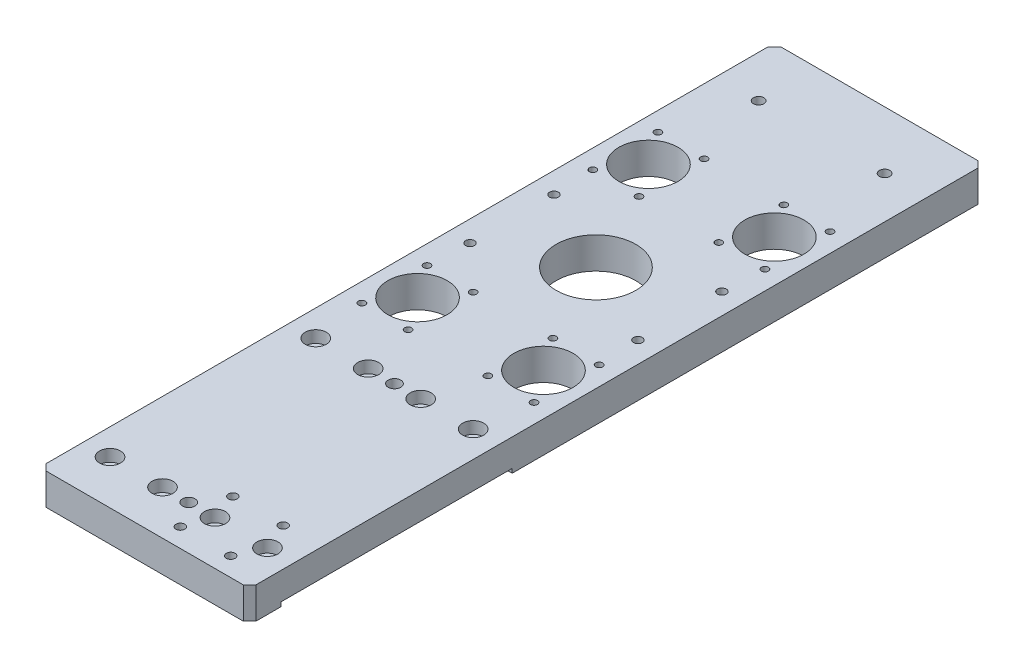
SolidWorks part; units mm, degrees
material "A6061 T6"
ref_plane "前视基准面" through (0, 0, 0) normal (0, 0, 1) x (1, 0, 0)
ref_plane "上视基准面" through (0, 0, 0) normal (0, 1, 0) x (1, 0, 0)
ref_plane "右视基准面" through (0, 0, 0) normal (1, 0, 0) x (0, 0, -1)
sketch "草图1" plane through (0, 0, 0) normal (0, 1, 0) x (1, 0, 0)
  line L1 (-50, 175) -> (50, 175)
  line L2 (-50, 175) -> (-50, -175)
  line L3 (-50, -175) -> (50, -175)
  line L4 (50, 175) -> (50, -175)
  line L5 (-50, 175) -> (50, -175) construction
  line L6 (-50, -175) -> (50, 175) construction
  point P0 (0, 0)
  dimension "D1" = 100
  dimension "D2" = 350
extrude "凸台-拉伸1" add sketch "草图1" along normal blind 15
sketch "草图3" plane through (0, 0, 0) normal (0, -1, 0) x (1, 0, 0)
  line L0 (-50, -175) -> (-50, 175) construction
  line L1 (-50, 160.1) -> (50, 160.1)
  line L2 (-50, 160.1) -> (-50, 49.9)
  line L3 (-50, 49.9) -> (50, 49.9)
  line L4 (50, 160.1) -> (50, 49.9)
  line L5 (50, 175) -> (50, -175) construction
  line L6 (-50, 175) -> (50, 175) construction
  dimension "D1" = 14.9
  dimension "D2" = 110.2
extrude "切除-拉伸1" cut sketch "草图3" against normal blind 2
hole_wizard "打孔尺寸(%根据)内六角圆柱头螺钉的类型1" positions "草图4" profile "草图5" counterbore size "M5" standard "GB"
sketch "草图4" plane through (0, 15, 0) normal (0, 1, 0) x (1, 0, 0)
  point P0 (-37.5, -154)
  point P3 (-12.5, -154)
  point P6 (12.5, -154)
  point P9 (37.5, -154)
  point P12 (-37.5, -56)
  point P15 (-12.5, -56)
  point P18 (12.5, -56)
  point P21 (37.5, -56)
sketch "草图5" plane through (-37.5, 15, 154) normal (1, 0, 0) x (0, 0, 1)
  line L0 (0, 0) -> (0, 16.6524)
  line L1 (0, 16.6524) -> (2.75, 15)
  line L2 (2.75, 15) -> (2.75, 5.7)
  line L3 (2.75, 5.7) -> (5, 5.7)
  line L4 (5, 5.7) -> (5, 0)
  line L5 (5, 0) -> (0, 0)
  line L10 (0, 16.6524) -> (-2.75, 15) construction
  line L11 (0, -6.35) -> (0, 107.95) construction
  dimension "孔直径" = 5.5
  dimension "孔深度" = 15
  dimension "柱形沉头孔直径" = 10
  dimension "柱形沉头孔深度" = 5.7
  dimension "导头角度" = 118
hole_wizard "大小mm 暗销孔1" positions "草图6" profile "草图7" hole size "Ø6.0" standard "GB"
sketch "草图6" plane through (0, 15, 0) normal (0, 1, 0) x (1, 0, 0)
  point P2 (0, -154)
  point P5 (0, -56)
sketch "草图7" plane through (0, 15, 154) normal (1, 0, 0) x (0, 0, 1)
  line L0 (0, 0) -> (0, 16.8026)
  line L1 (0, 16.8026) -> (3, 15)
  line L2 (3, 15) -> (3, 0)
  line L5 (3, 0) -> (0, 0)
  line L10 (0, 16.8026) -> (-3, 15) construction
  line L11 (0, -6.35) -> (0, 107.95) construction
  dimension "孔直径" = 6
  dimension "孔深度" = 15
  dimension "导头角度" = 118
sketch "草图8" plane through (0, 15, 0) normal (0, 1, 0) x (1, 0, 0)
  line L0 (-50, 175) -> (-50, -175) construction
  line L1 (50, 175) -> (-50, 175) construction
  circle A0 centre (0, 40) radius 19
  dimension "D1" = 38
  dimension "D2" = 50
  dimension "D3" = 135
extrude "切除-拉伸2" cut sketch "草图8" against normal blind 20
chamfer "倒角1" distance 3 angle 45 4 edges at (50, 7.5, -175) (-50, 7.5, -175) (50, 7.5, 175) (-50, 7.5, 175)
sketch "草图9" plane through (0, 15, 0) normal (0, 1, 0) x (1, 0, 0)
  line L0 (47, 175) -> (-47, 175) construction
  line L1 (50, -172) -> (50, 172) construction
  line L2 (-50, 172) -> (-50, -172) construction
  circle A0 centre (30, -15) radius 14.1
  circle A1 centre (30, 95) radius 14.1
  circle A3 centre (-30, -15) radius 14.1
  circle A4 centre (-30, 95) radius 14.1
  dimension "D1" = 80
  dimension "D2" = 110
  dimension "D3" = 28.2
  dimension "D4" = 20
  dimension "D5" = 28.2
  dimension "D6" = 20
extrude "切除-拉伸3" cut sketch "草图9" against normal blind 20
hole_wizard "大小mm 暗销孔2" positions "草图14" profile "草图15" hole size "Ø5.0" standard "GB"
sketch "草图14" plane through (0, 15, 0) normal (0, 1, 0) x (1, 0, 0)
  point P0 (30, 147.5)
  point P3 (-30, 147.5)
sketch "草图15" plane through (30, 15, -147.5) normal (1, 0, 0) x (0, 0, 1)
  line L0 (0, 0) -> (0, 21.5022)
  line L1 (0, 21.5022) -> (2.5, 20)
  line L2 (2.5, 20) -> (2.5, 0)
  line L5 (2.5, 0) -> (0, 0)
  line L10 (0, 21.5022) -> (-2.5, 20) construction
  line L11 (0, -6.35) -> (0, 107.95) construction
  dimension "孔直径" = 5
  dimension "孔深度" = 20
  dimension "导头角度" = 118
hole_wizard "M5 螺纹孔1" positions "草图18" profile "草图19" tap size "M5" standard "GB"
sketch "草图18" plane through (0, 0, 0) normal (0, -1, 0) x (-1, 0, 0)
  point P0 (40, 20)
  point P3 (-40, 20)
  point P6 (40, 60)
  point P9 (-40, 60)
sketch "草图19" plane through (-40, 0, -20) normal (1, 0, 0) x (0, 0, -1)
  line L0 (0, 0) -> (0, 21.2618)
  line L1 (0, 21.2618) -> (2.1, 20)
  line L2 (2.1, 20) -> (2.1, 0)
  line L5 (2.1, 0) -> (0, 0)
  line L10 (0, 21.2618) -> (-2.1, 20) construction
  line L11 (0, -6.35) -> (0, 107.95) construction
  dimension "螺纹孔钻头直径" = 4.2
  dimension "螺纹孔钻头深度" = 20
  dimension "导头角度" = 118
cosmetic thread "孔螺蚊线5" parameters "D1"=10, "D2"=5
cosmetic thread "孔螺蚊线6" parameters "D1"=10, "D2"=5
cosmetic thread "孔螺蚊线7" parameters "D1"=10, "D2"=5
cosmetic thread "孔螺蚊线8" parameters "D1"=10, "D2"=5
hole_wizard "M4 螺纹孔1" positions "草图20" profile "草图21" tap size "M4" standard "GB"
sketch "草图20" plane through (0, 15, 0) normal (0, 1, 0) x (1, 0, 0)
  point P0 (41, -30.5)
  point P3 (19, -30.5)
  point P6 (41, 0.5)
  point P9 (19, 0.5)
  point P12 (-19, -30.5)
  point P15 (-41, -30.5)
  point P18 (-19, 0.5)
  point P21 (-41, 0.5)
  point P24 (41, 79.5)
  point P27 (19, 79.5)
  point P30 (41, 110.5)
  point P33 (19, 110.5)
  point P36 (-19, 79.5)
  point P39 (-41, 79.5)
  point P42 (-19, 110.5)
  point P45 (-41, 110.5)
sketch "草图21" plane through (41, 15, 30.5) normal (1, 0, 0) x (0, 0, 1)
  line L0 (0, 0) -> (0, 32.9914)
  line L1 (0, 32.9914) -> (1.65, 32)
  line L2 (1.65, 32) -> (1.65, 0)
  line L5 (1.65, 0) -> (0, 0)
  line L10 (0, 32.9914) -> (-1.65, 32) construction
  line L11 (0, -6.35) -> (0, 107.95) construction
  dimension "螺纹孔钻头直径" = 3.3
  dimension "螺纹孔钻头深度" = 32
  dimension "导头角度" = 118
cosmetic thread "孔螺蚊线9" parameters "D1"=8, "D2"=4
cosmetic thread "孔螺蚊线10" parameters "D1"=8, "D2"=4
cosmetic thread "孔螺蚊线11" parameters "D1"=8, "D2"=4
cosmetic thread "孔螺蚊线12" parameters "D1"=8, "D2"=4
cosmetic thread "孔螺蚊线13" parameters "D1"=8, "D2"=4
cosmetic thread "孔螺蚊线14" parameters "D1"=8, "D2"=4
cosmetic thread "孔螺蚊线15" parameters "D1"=8, "D2"=4
cosmetic thread "孔螺蚊线16" parameters "D1"=8, "D2"=4
cosmetic thread "孔螺蚊线17" parameters "D1"=8, "D2"=4
cosmetic thread "孔螺蚊线18" parameters "D1"=8, "D2"=4
cosmetic thread "孔螺蚊线19" parameters "D1"=8, "D2"=4
cosmetic thread "孔螺蚊线20" parameters "D1"=8, "D2"=4
cosmetic thread "孔螺蚊线21" parameters "D1"=8, "D2"=4
cosmetic thread "孔螺蚊线22" parameters "D1"=8, "D2"=4
cosmetic thread "孔螺蚊线23" parameters "D1"=8, "D2"=4
cosmetic thread "孔螺蚊线24" parameters "D1"=8, "D2"=4
hole_wizard "M5 螺纹孔2" positions "草图22" profile "草图23" tap size "M5" standard "GB"
sketch "草图22" plane through (0, 15, 0) normal (0, 1, 0) x (1, 0, 0)
  point P0 (8, -141)
  point P3 (32, -141)
  point P6 (8, -166)
  point P9 (32, -166)
sketch "草图23" plane through (8, 15, 141) normal (1, 0, 0) x (0, 0, 1)
  line L0 (0, 0) -> (0, 21.2618)
  line L1 (0, 21.2618) -> (2.1, 20)
  line L2 (2.1, 20) -> (2.1, 0)
  line L5 (2.1, 0) -> (0, 0)
  line L10 (0, 21.2618) -> (-2.1, 20) construction
  line L11 (0, -6.35) -> (0, 107.95) construction
  dimension "螺纹孔钻头直径" = 4.2
  dimension "螺纹孔钻头深度" = 20
  dimension "导头角度" = 118
cosmetic thread "孔螺蚊线25" parameters "D1"=10, "D2"=5
cosmetic thread "孔螺蚊线26" parameters "D1"=10, "D2"=5
cosmetic thread "孔螺蚊线27" parameters "D1"=10, "D2"=5
cosmetic thread "孔螺蚊线28" parameters "D1"=10, "D2"=5
